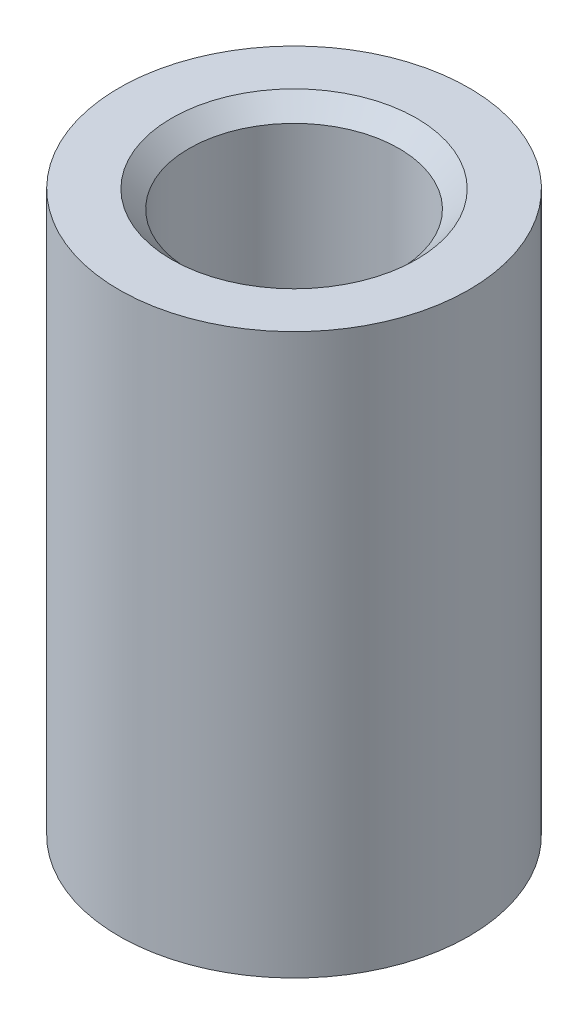
SolidWorks part; units mm, degrees
material "Plain Carbon Steel"
ref_plane "Front Plane" through (0, 0, 0) normal (0, 0, 1) x (1, 0, 0)
ref_plane "Top Plane" through (0, 0, 0) normal (0, 1, 0) x (1, 0, 0)
ref_plane "Right Plane" through (0, 0, 0) normal (1, 0, 0) x (0, 0, -1)
sketch "Sketch1" plane through (0, 0, 0) normal (0, 0, 1) x (1, 0, 0)
  line L0 (0, -264.3045) -> (0, 12950.9186) construction
  line L1 (0, 0) -> (5, 0)
  line L2 (5, 0) -> (5, -16)
  line L3 (5, -16) -> (0, -16)
  line L4 (0, -16) -> (0, 0)
  dimension "D1" = 5
  dimension "D2" = 16
revolve "Revolve1" add sketch "Sketch1" angle 360 about L0
sketch "Sketch2" plane through (0, 0, 0) normal (0, 1, 0) x (1, 0, 0)
  circle A0 centre (0, 0) radius 3
  dimension "D1" = 6
extrude "Cut-Extrude1" cut sketch "Sketch2" against normal blind 10
chamfer "Chamfer1" distance 0.5 angle 45 1 edges at (-3, 0, 0)
